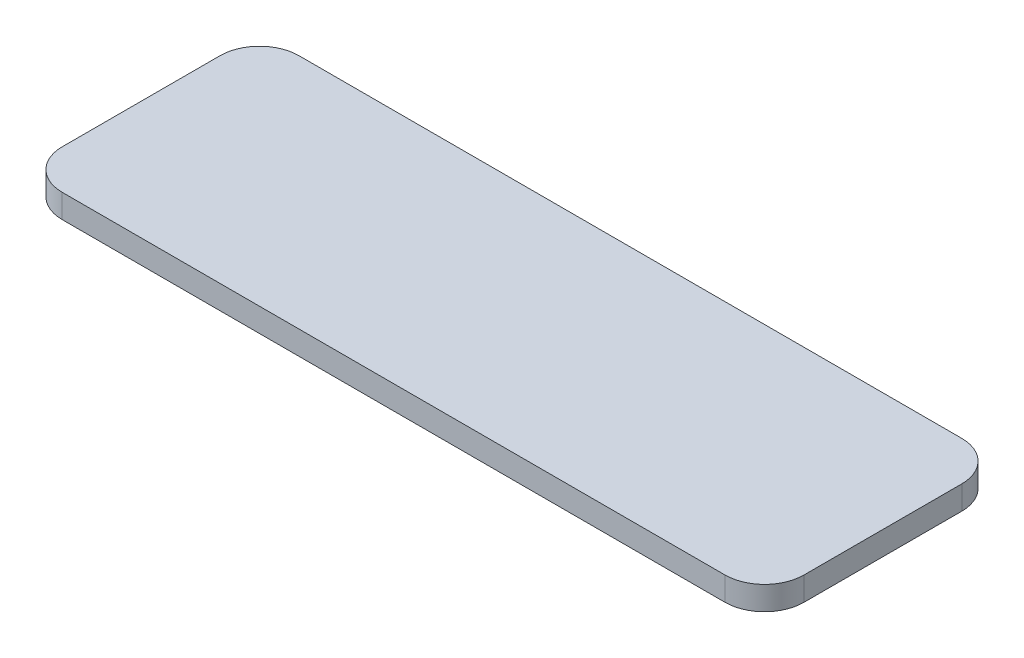
SolidWorks part; units mm, degrees
ref_plane "Front Plane" through (0, 0, 0) normal (0, 0, 1) x (1, 0, 0)
ref_plane "Top Plane" through (0, 0, 0) normal (0, 1, 0) x (1, 0, 0)
ref_plane "Right Plane" through (0, 0, 0) normal (1, 0, 0) x (0, 0, -1)
sketch "Sketch1" plane through (0, 0, 0) normal (0, 1, 0) x (1, 0, 0)
  line L1 (-47, -15) -> (47, -15)
  line L2 (-47, -15) -> (-47, 15)
  line L3 (-47, 15) -> (47, 15)
  line L4 (47, -15) -> (47, 15)
  line L5 (-47, -15) -> (47, 15) construction
  line L6 (-47, 15) -> (47, -15) construction
  point P0 (0, 0)
  dimension "D1" = 94
  dimension "D2" = 30
extrude "Boss-Extrude1" add sketch "Sketch1" along normal blind 3
fillet "Fillet1" radius 5 4 edges at (47, 1.5, 15) (47, 1.5, -15) (-47, 1.5, -15) (-47, 1.5, 15)
